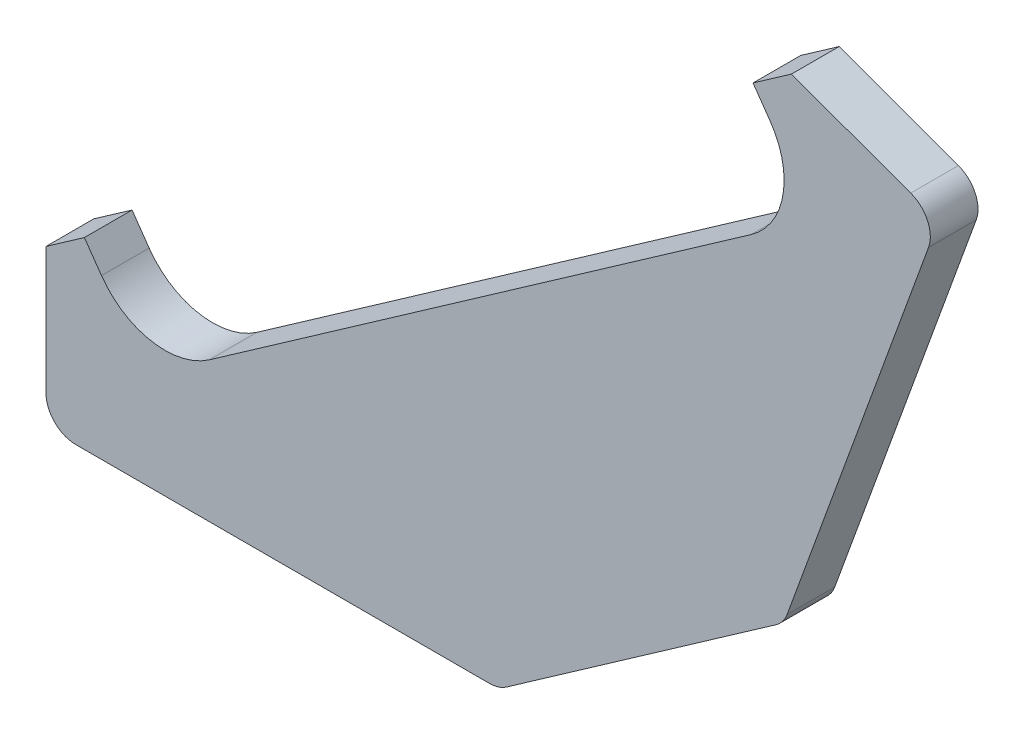
SolidWorks part; units mm, degrees
material "Q235-A "
ref_plane "前视基准面" through (0, 0, 0) normal (0, 0, 1) x (1, 0, 0)
ref_plane "上视基准面" through (0, 0, 0) normal (0, 1, 0) x (1, 0, 0)
ref_plane "右视基准面" through (0, 0, 0) normal (1, 0, 0) x (0, 0, -1)
sketch "草图1" plane through (0, 0, 0) normal (0, 0, 1) x (1, 0, 0)
  line L0 (-132, 141.9017) -> (-152, 141.9017)
  line L1 (-132, 141.9017) -> (-132, 177.8054) construction
  line L2 (-132, 141.9017) -> (0, 141.9017)
  line L3 (0, 141.9017) -> (95.6883, 208.9033)
  line L4 (95.6883, 208.9033) -> (140.8349, 332.9427)
  line L5 (160.161, 325.9086) -> (140.8349, 332.9427) construction
  line L6 (140.8349, 332.9427) -> (130.5743, 304.752) construction
  line L7 (85.3397, 360.7055) -> (91.0755, 352.5139)
  line L8 (-97.1613, 188.969) -> (84.6905, 316.303)
  line L9 (-152, 141.9017) -> (-152, 194.5184)
  line L10 (-152, 182.3107) -> (-133.3722, 195.354) construction
  line L11 (-6.2354, 252.636) -> (64.2158, 152.0213) construction
  line L12 (109.7033, 365.5573) -> (91.0755, 352.5139) construction
  line L14 (140.8349, 332.9427) -> (147.6753, 351.7366)
  line L15 (-133.3722, 195.354) -> (-139.108, 203.5455)
  line L16 (85.3397, 360.7055) -> (98.2317, 369.7326)
  line L18 (-139.108, 203.5455) -> (-152, 194.5184)
  line L19 (147.6753, 351.7366) -> (98.2317, 369.7326)
  arc A4 (-133.3722, 195.354) -> (-97.1613, 188.969) centre (-112.0742, 210.267) ccw construction
  arc A5 (-133.3722, 195.354) -> (-97.1613, 188.969) centre (-112.0742, 210.267) ccw
  arc A6 (84.6905, 316.303) -> (91.0755, 352.5139) centre (69.7775, 337.601) ccw construction
  arc A7 (84.6905, 316.303) -> (91.0755, 352.5139) centre (69.7775, 337.601) ccw
  dimension "D1" = 20
  dimension "D2" = 10
extrude "凸台-拉伸1" add sketch "草图1" along normal blind 16
fillet "圆角1" radius 10 4 edges at (0, 141.9017, 8) (95.6883, 208.9033, 8) (-152, 141.9017, 8) (147.6753, 351.7366, 8)
